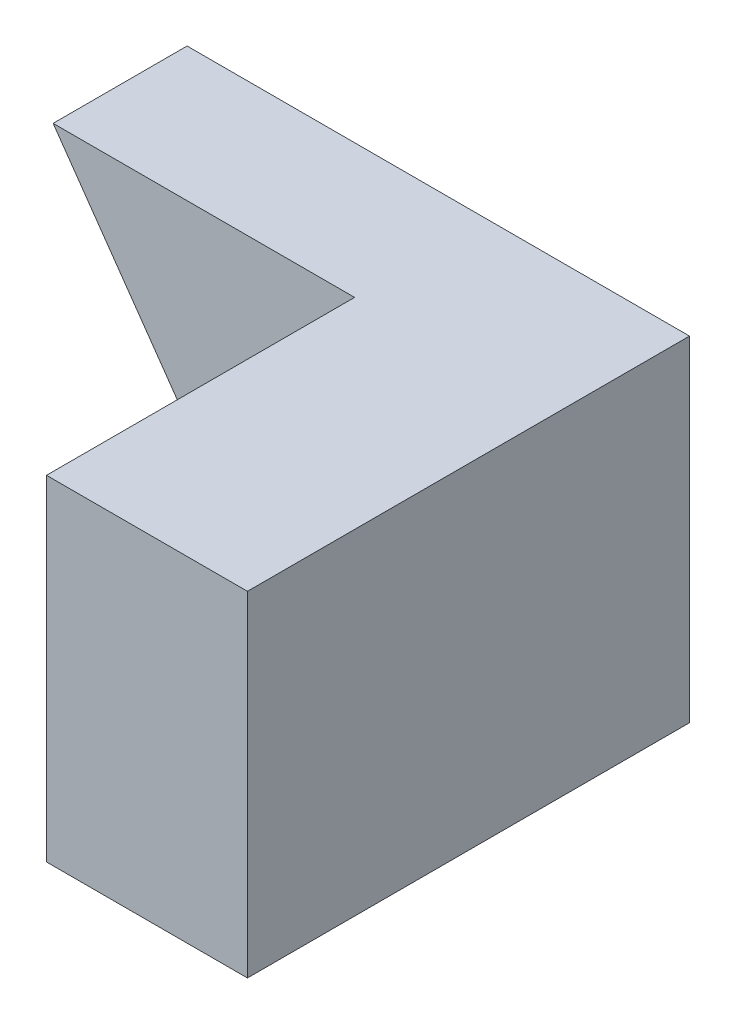
from build123d import *

# Parameters (mm, degrees)
BOSS_EXTRUDE1_DEPTH = 1
SKETCH2_W           = 1.5
SKETCH2_H           = 2.5
BOSS_EXTRUDE2_DEPTH = 2.3


with BuildPart() as part:
    # Sketch1 → Boss-Extrude1 (new body)
    with BuildSketch(Plane.XY):
        Polygon((0, 0), (-1.750518846, 2.5), (2, 2.5), (2, 0), align=None)
    extrude(amount=BOSS_EXTRUDE1_DEPTH)

    # Sketch2 → Boss-Extrude2 (add)
    with BuildSketch(Plane.XY.offset(1)):
        with Locations((1.25, 1.25)):
            Rectangle(SKETCH2_W, SKETCH2_H)
    extrude(amount=BOSS_EXTRUDE2_DEPTH)


solid = part.part
